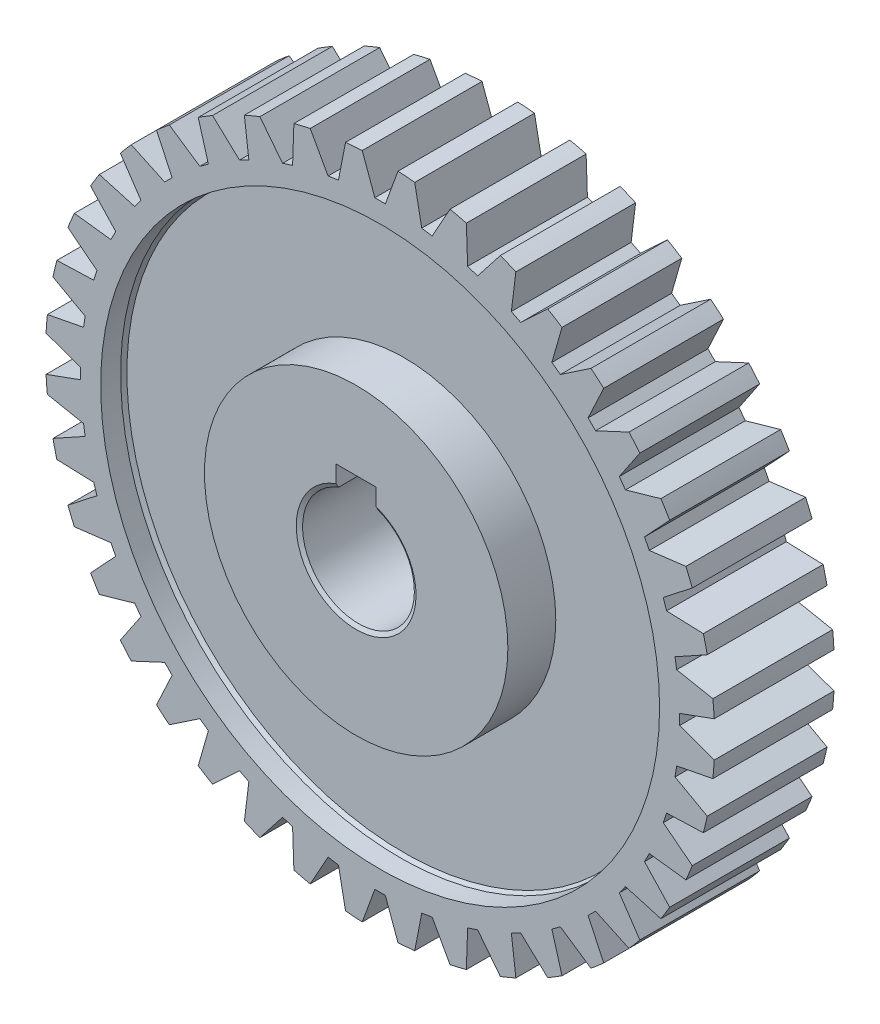
SolidWorks part; units mm, degrees
ref_plane "Front Plane" through (0, 0, 0) normal (0, 0, 1) x (1, 0, 0)
ref_plane "Top Plane" through (0, 0, 0) normal (0, 1, 0) x (1, 0, 0)
ref_plane "Right Plane" through (0, 0, 0) normal (1, 0, 0) x (0, 0, -1)
other "Configuration Table"
sketch "Sketch1" plane through (0, 0, 0) normal (0, 0, 1) x (1, 0, 0)
  circle A0 centre (0, 0) radius 41.895
  dimension "D1" = 83.79
extrude "Boss-Extrude1" add sketch "Sketch1" along normal blind 15
sketch "Sketch2" plane through (0, 0, 0) normal (0, 0, -1) x (-1, 0, 0)
  circle A0 centre (0, 0) radius 12
  dimension "D1" = 24
extrude "Boss-Extrude2" add sketch "Sketch2" along normal blind 3
sketch "Sketch3" plane through (0, 0, 15) normal (0, 0, 1) x (1, 0, 0)
  circle A0 centre (0, 0) radius 19
  circle A1 centre (0, 0) radius 35
  dimension "D1" = 70
  dimension "D2" = 38
extrude "Cut-Extrude1" cut sketch "Sketch3" against normal blind 3
sketch "Sketch4" plane through (0, 0, 15) normal (0, 0, 1) x (1, 0, 0)
  circle A1 centre (0, 0) radius 19
  circle A2 centre (0, 0) radius 19
  dimension "D1" = 0
extrude "Boss-Extrude3" add sketch "Sketch4" along normal blind 3
sketch "Sketch5" plane through (0, 0, 18) normal (0, 0, 1) x (1, 0, 0)
  line L1 (-2.5, 9.2) -> (2.5, 9.2)
  line L2 (-2.5, 9.2) -> (-2.5, 4.8)
  line L3 (-2.5, 4.8) -> (2.5, 4.8)
  line L4 (2.5, 9.2) -> (2.5, 4.8)
  line L5 (-2.5, 9.2) -> (2.5, 4.8) construction
  line L6 (-2.5, 4.8) -> (2.5, 9.2) construction
  circle A0 centre (0, 0) radius 7
  point P3 (0, 7)
  dimension "D1" = 14
  dimension "D2" = 9.2
  dimension "D3" = 5
extrude "Cut-Extrude2" cut sketch "Sketch5" against normal through all contours A0 L4 L1 L2 | L4 A0 L2 L3 | L2 A0 L4 L3
sketch "Sketch6" plane through (0, 0, 0) normal (0, 0, 1) x (1, 0, 0)
  line L0 (0, 54.0275) -> (0, 0) construction
  line L1 (0.6601, 37.5) -> (-0.6601, 37.5)
  line L2 (-0.6601, 37.5) -> (-3.235, 44.5746)
  line L3 (-3.235, 44.5746) -> (3.235, 44.5746)
  line L4 (-1.57, 40) -> (1.57, 40) construction
  line L5 (0.6601, 37.5) -> (3.235, 44.5746)
  point P10 (0, 40)
  point P11 (0, 44.5746)
  point P12 (0, 37.5)
  dimension "D1" = 20
  dimension "D2" = 3.14
  dimension "D3" = 2.5
  dimension "D4" = 40
extrude "Cut-Extrude3" cut sketch "Sketch6" along normal blind 26
pattern_circular "CirPattern1" count 40 over 360 about axis through (0, 0, 0) along (0, 0, 1) of "Cut-Extrude3"
chamfer "Chamfer1" distance 0.5 angle 30 2 edges at (0, -7, -3) (0, -7, 18)
chamfer "Chamfer2" distance 0.5 angle 30 1 edges at (35, 0, 12)
